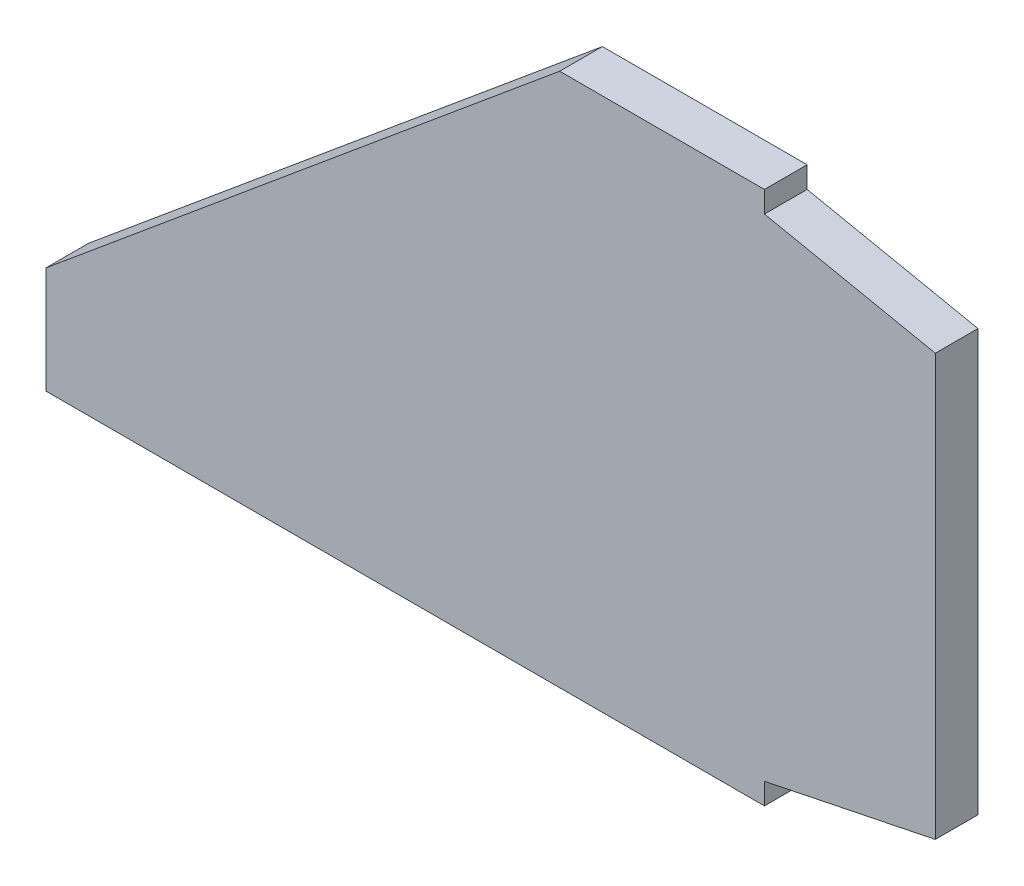
from build123d import *

# Parameters (mm, degrees)
BOSS_EXTRUDE1_DEPTH = 20


with BuildPart() as part:
    # Sketch1 → Boss-Extrude1 (new body)
    with BuildSketch(Plane.XY):
        Polygon((15783.129958129, 4624.359704887), (15687.257317346, 4624.359704887), (15446.728394371, 4424.359704449), (15446.728394371, 4374.359704887), (15783.129958129, 4374.359704887), (15783.129958129, 4384.359705726), (15863.129958392, 4400.769556521), (15863.129958392, 4597.949855679), (15783.129958129, 4614.359706473), align=None)
    extrude(amount=BOSS_EXTRUDE1_DEPTH)


solid = part.part
